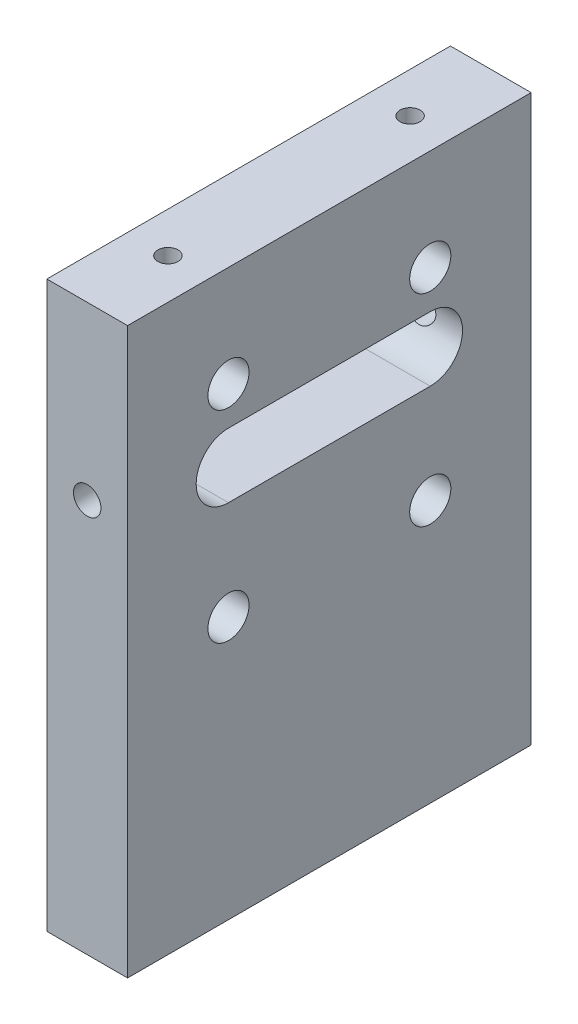
SolidWorks part; units mm, degrees
ref_plane "前视基准面" through (0, 0, 0) normal (0, 0, 1) x (1, 0, 0)
ref_plane "上视基准面" through (0, 0, 0) normal (0, 1, 0) x (1, 0, 0)
ref_plane "右视基准面" through (0, 0, 0) normal (1, 0, 0) x (0, 0, -1)
sketch "草图1" plane through (0, 0, 0) normal (1, 0, 0) x (0, 0, -1)
  line L1 (-50, 70) -> (50, 70)
  line L2 (-50, 70) -> (-50, -70)
  line L3 (-50, -70) -> (50, -70)
  line L4 (50, 70) -> (50, -70)
  line L5 (-50, 70) -> (50, -70) construction
  line L6 (-50, -70) -> (50, 70) construction
  point P0 (0, 0)
  dimension "D1" = 100
  dimension "D2" = 140
extrude "凸台-拉伸1" add sketch "草图1" along normal blind 20
hole_wizard "M6 螺纹孔1" positions "草图2" profile "草图3" tap size "M6" standard "GB"
sketch "草图2" plane through (0, -70, 0) normal (0, -1, 0) x (-1, 0, 0)
  line L0 (-10, -50) -> (-10, 47.319) construction
  line L1 (-20, -50) -> (0, -50) construction
  line L3 (0, 0) -> (-16.4512, 0) construction
  point P0 (-10, 30)
  point P2 (-10, -30)
  dimension "D1" = 60
sketch "草图3" plane through (10, -70, -30) normal (1, 0, 0) x (0, 0, -1)
  line L0 (0, 0) -> (0, 16.5022)
  line L1 (0, 16.5022) -> (2.5, 15)
  line L2 (2.5, 15) -> (2.5, 0)
  line L5 (2.5, 0) -> (0, 0)
  line L10 (0, 16.5022) -> (-2.5, 15) construction
  line L11 (0, -6.35) -> (0, 107.95) construction
  dimension "螺纹孔钻头直径" = 5
  dimension "螺纹孔钻头深度" = 15
  dimension "导头角度" = 118
cosmetic thread "孔螺蚊线1" parameters "D1"=12, "D2"=6
cosmetic thread "孔螺蚊线2" parameters "D1"=12, "D2"=6
sketch "草图4" plane through (0, 0, 0) normal (-1, 0, 0) x (0, 0, 1)
  line L0 (-25, 27.5) -> (25, 27.5) construction
  line L1 (-25, 35.5) -> (25, 35.5)
  line L2 (-25, 19.5) -> (25, 19.5)
  line L3 (0, -70) -> (0, 43.5925) construction
  line L4 (50, -70) -> (-50, -70) construction
  arc A0 (-25, 35.5) -> (-25, 19.5) centre (-25, 27.5) ccw
  arc A1 (25, 19.5) -> (25, 35.5) centre (25, 27.5) ccw
  point P2 (0, 27.5)
  dimension "D1" = 16
  dimension "D2" = 50
  dimension "D3" = 97.5
extrude "切除-拉伸1" cut sketch "草图4" against normal through all
hole_wizard "M8 螺纹孔1" positions "草图5" profile "草图6" tap size "M8" standard "GB" end condition through all
sketch "草图5" plane through (0, 0, 50) normal (0, 0, 1) x (1, 0, 0)
  line L0 (0, 35.5) -> (0, 19.5) construction
  line L2 (0, 27.5) -> (26.2444, 27.5) construction
  line L4 (10, 70) -> (10, 5.2092) construction
  line L5 (20, 70) -> (0, 70) construction
  point P0 (10, 27.5)
sketch "草图6" plane through (10, 27.5, 50) normal (1, 0, 0) x (0, -1, 0)
  line L0 (0, 0) -> (0, 100)
  line L1 (0, 100) -> (3.4, 100)
  line L2 (3.4, 100) -> (3.4, 0)
  line L5 (3.4, 0) -> (0, 0)
  line L11 (0, -6.35) -> (0, 107.95) construction
  dimension "通孔螺纹孔钻头直径" = 6.8
  dimension "通孔螺纹孔钻头深度" = 100
cosmetic thread "孔螺蚊线3" parameters "D2"=8
hole_wizard "M12 螺纹孔1" positions "草图7" profile "草图8" tap size "M12" standard "GB" end condition through all
sketch "草图7" plane through (0, 0, 0) normal (-1, 0, 0) x (0, 0, 1)
  line L0 (0, -70) -> (0, 87.4043) construction
  line L1 (50, -70) -> (-50, -70) construction
  point P0 (-25, 45)
  point P2 (25, 45)
  point P4 (-25, -5)
  point P6 (25, -5)
  dimension "D3" = 50
  dimension "D1" = 50
  dimension "D2" = 65
sketch "草图8" plane through (0, 45, -25) normal (0, 1, 0) x (0, 0, 1)
  line L0 (0, 0) -> (0, 20)
  line L1 (0, 20) -> (5.1, 20)
  line L2 (5.1, 20) -> (5.1, 0.925)
  line L3 (5.1, 0.925) -> (6.025, 0)
  line L5 (6.025, 0) -> (0, 0)
  line L6 (-5.1, 0.925) -> (-6.025, 0) construction
  line L11 (0, -6.35) -> (0, 107.95) construction
  dimension "通孔螺纹孔钻头直径" = 10.2
  dimension "通孔螺纹孔钻头深度" = 20
  dimension "近端锥形沉头孔直径" = 12.05
  dimension "近端锥形沉头孔角度" = 90
cosmetic thread "孔螺蚊线4" parameters "D2"=12
cosmetic thread "孔螺蚊线5" parameters "D2"=12
cosmetic thread "孔螺蚊线6" parameters "D2"=12
cosmetic thread "孔螺蚊线7" parameters "D2"=12
hole_wizard "M6 螺纹孔2" positions "草图9" profile "草图10" tap size "M6" standard "GB"
sketch "草图9" plane through (0, 70, 0) normal (0, 1, 0) x (1, 0, 0)
  line L0 (10, -50) -> (10, 57.0642) construction
  line L1 (20, -50) -> (0, -50) construction
  line L3 (0, 0) -> (32.5571, 0) construction
  point P0 (10, 30)
  point P2 (10, -30)
  dimension "D1" = 60
sketch "草图10" plane through (10, 70, -30) normal (1, 0, 0) x (0, 0, 1)
  line L0 (0, 0) -> (0, 16.5022)
  line L1 (0, 16.5022) -> (2.5, 15)
  line L2 (2.5, 15) -> (2.5, 0)
  line L5 (2.5, 0) -> (0, 0)
  line L10 (0, 16.5022) -> (-2.5, 15) construction
  line L11 (0, -6.35) -> (0, 107.95) construction
  dimension "螺纹孔钻头直径" = 5
  dimension "螺纹孔钻头深度" = 15
  dimension "导头角度" = 118
cosmetic thread "孔螺蚊线8" parameters "D1"=12, "D2"=6
cosmetic thread "孔螺蚊线9" parameters "D1"=12, "D2"=6
